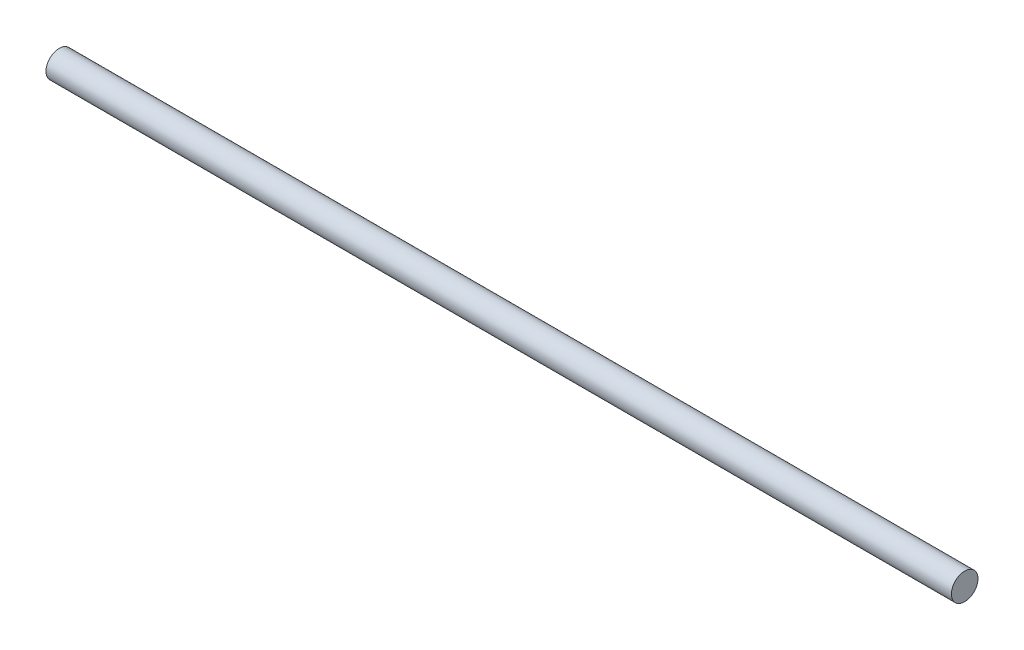
SolidWorks part; units mm, degrees
material "Q235A"
ref_plane "前视基准面" through (0, 0, 0) normal (0, 0, 1) x (1, 0, 0)
ref_plane "上视基准面" through (0, 0, 0) normal (0, 1, 0) x (1, 0, 0)
ref_plane "右视基准面" through (0, 0, 0) normal (1, 0, 0) x (0, 0, -1)
sketch "草图1" plane through (0, 0, 0) normal (0, 0, 1) x (1, 0, 0)
  line L0 (0, 0) -> (1021.5, 0)
  dimension "D1" = 1021.5
other "圆管 30X3(1)"
ref_plane "基准面1" through (0, 0, 0) normal (1, 0, 0) x (0, 1, 0)
sketch "Sketch12" plane through (0, 0, 0) normal (1, 0, 0) x (0, 1, 0)
  circle A0 centre (0, 0) radius 12
  circle A1 centre (0, 0) radius 15
  point P3 (0, 0)
  dimension "Out_dia" = 30
  dimension "D1" = 3
sketch "草图3" plane through (0, 0, 0) normal (-1, 0, 0) x (0, 0, 1)
  circle A0 centre (0, 0) radius 14
  circle A1 centre (0, 0) radius 15
  circle A2 centre (0, 0) radius 15
  dimension "D1" = 0
  dimension "D2" = 1
extrude "切除-拉伸1" [suppressed] cut sketch "草图3" against normal blind 30
sketch "草图4" plane through (1021.5, 0, 0) normal (1, 0, 0) x (0, 0, -1)
  circle A1 centre (0, 0) radius 15
  circle A2 centre (0, 0) radius 15
  circle A3 centre (0, 0) radius 14
  circle A4 centre (0, 0) radius 14
  dimension "D1" = 0
  dimension "D2" = 0
extrude "切除-拉伸2" [suppressed] cut sketch "草图4" against normal blind 30
sketch "草图5" plane through (1021.5, 0, 0) normal (1, 0, 0) x (0, 0, -1)
  circle A0 centre (0, 0) radius 12 construction
  circle A1 centre (0, 0) radius 12
extrude "凸台-拉伸2" add sketch "草图5" against normal through all
